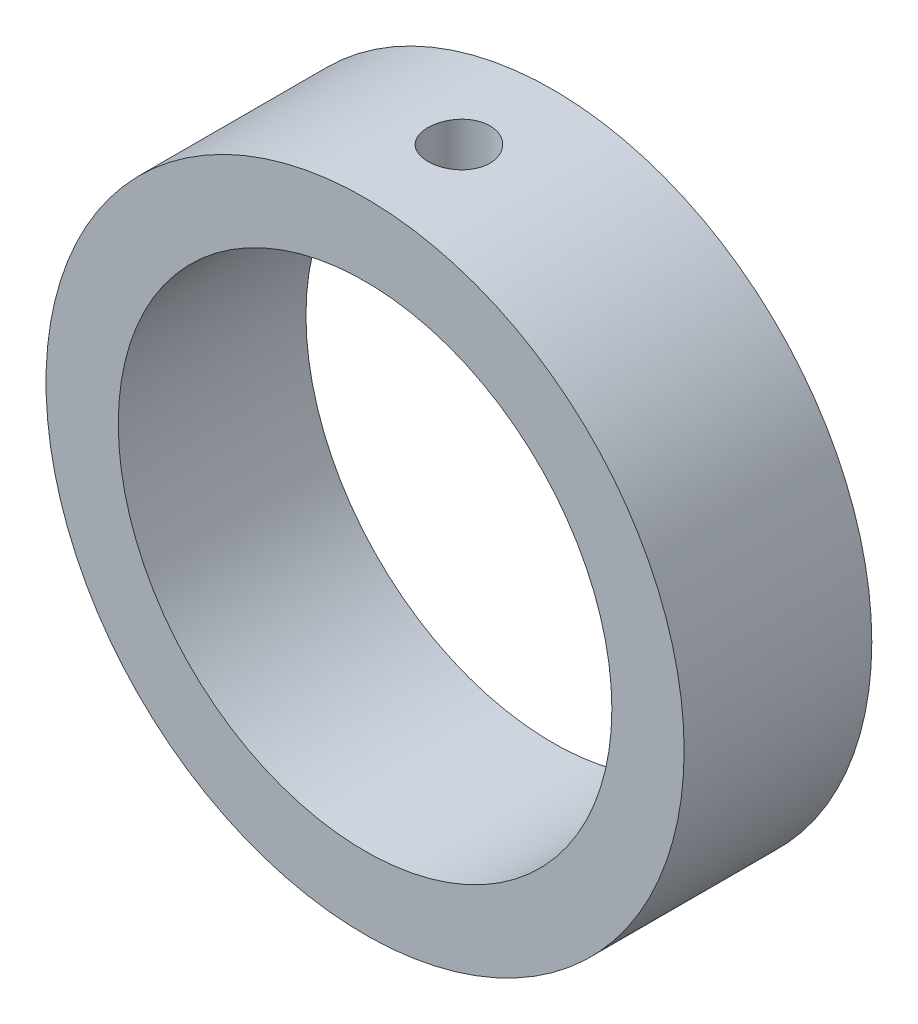
SolidWorks part; units mm, degrees
ref_plane "前视基准面" through (0, 0, 0) normal (0, 0, 1) x (1, 0, 0)
ref_plane "上视基准面" through (0, 0, 0) normal (0, 1, 0) x (1, 0, 0)
ref_plane "右视基准面" through (0, 0, 0) normal (1, 0, 0) x (0, 0, -1)
sketch "草图1" plane through (0, 0, 0) normal (0, 0, 1) x (1, 0, 0)
  circle A0 centre (0, 0) radius 13.15
  circle A1 centre (0, 0) radius 17
  dimension "D1" = 26.3
  dimension "D2" = 34
extrude "凸台-拉伸1" add sketch "草图1" along normal mid plane 10
hole_wizard "M4 螺纹孔2" positions "草图7" profile "草图8" tap size "M4" standard "GB"
sketch "草图7" plane through (0, 0, 0) normal (0, 1, 0) x (1, 0, 0)
  point P0 (0, 0)
sketch "草图8" plane through (0, 0, 0) normal (1, 0, 0) x (0, 0, -1)
  line L0 (0, 0) -> (0, 17)
  line L1 (0, 17) -> (1.65, 17)
  line L2 (1.65, 17) -> (1.65, 0)
  line L5 (1.65, 0) -> (0, 0)
  line L11 (0, -6.35) -> (0, 107.95) construction
  dimension "通孔螺纹孔钻头直径" = 3.3
  dimension "通孔螺纹孔钻头深度" = 17
cosmetic thread "孔螺蚊线3" parameters "D2"=4
